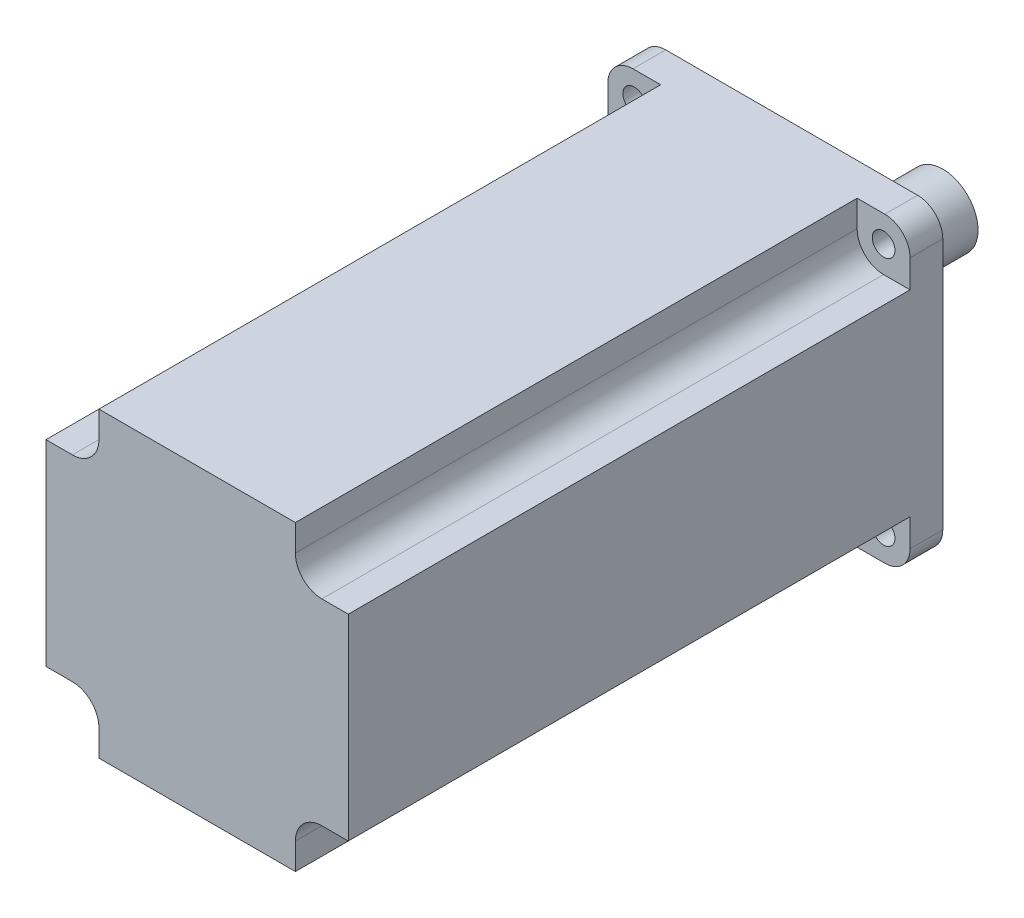
from build123d import *

# Parameters (mm, degrees)
SKETCH1_R      = 2.25
EXTRUDE1_DEPTH = 6.5
EXTRUDE2_DEPTH = 111.5
SKETCH3_R      = 25
EXTRUDE3_DEPTH = 3
SKETCH4_R      = 7
EXTRUDE4_DEPTH = 27


with BuildPart() as part:
    # Sketch1 → Extrude1 (new body)
    with BuildSketch(Plane.XY):
        with BuildLine():
            Line((-25, -30), (25, -30))
            ThreePointArc((25, -30), (28.535533906, -28.535533906), (30, -25))
            Line((30, -25), (30, 25))
            ThreePointArc((30, 25), (28.535533906, 28.535533906), (25, 30))
            Line((25, 30), (-25, 30))
            ThreePointArc((-25, 30), (-28.535533906, 28.535533906), (-30, 25))
            Line((-30, 25), (-30, -25))
            ThreePointArc((-30, -25), (-28.535533906, -28.535533906), (-25, -30))
        make_face()
        with Locations(Location((-24.748737342, 24.748737342, 0), (0, 0, 180))):
            Circle(SKETCH1_R, mode=Mode.SUBTRACT)
        with Locations(Location((-24.748737342, -24.748737342, 0), (0, 0, 180))):
            Circle(SKETCH1_R, mode=Mode.SUBTRACT)
        with Locations(Location((24.748737342, -24.748737342, 0), (0, 0, 180))):
            Circle(SKETCH1_R, mode=Mode.SUBTRACT)
        with Locations(Location((24.748737342, 24.748737342, 0), (0, 0, 180))):
            Circle(SKETCH1_R, mode=Mode.SUBTRACT)
    extrude(amount=EXTRUDE1_DEPTH)

    # Sketch2 → Extrude2 (add)
    with BuildSketch(Plane.XY.offset(6.5)):
        with BuildLine():
            Line((-19.497474683, -30), (19.497474683, -30))
            Line((19.497474683, -30), (19.497474683, -24.748737342))
            ThreePointArc((19.497474683, -24.748737342), (21.035533906, -21.035533906), (24.748737342, -19.497474683))
            Line((24.748737342, -19.497474683), (30, -19.497474683))
            Line((30, -19.497474683), (30, 19.497474683))
            Line((30, 19.497474683), (24.748737342, 19.497474683))
            ThreePointArc((24.748737342, 19.497474683), (21.035533906, 21.035533906), (19.497474683, 24.748737342))
            Line((19.497474683, 24.748737342), (19.497474683, 30))
            Line((19.497474683, 30), (-19.497474683, 30))
            Line((-19.497474683, 30), (-19.497474683, 24.748737342))
            ThreePointArc((-19.497474683, 24.748737342), (-21.035533906, 21.035533906), (-24.748737342, 19.497474683))
            Line((-24.748737342, 19.497474683), (-30, 19.497474683))
            Line((-30, 19.497474683), (-30, -19.497474683))
            Line((-30, -19.497474683), (-24.748737342, -19.497474683))
            ThreePointArc((-24.748737342, -19.497474683), (-21.035533906, -21.035533906), (-19.497474683, -24.748737342))
            Line((-19.497474683, -24.748737342), (-19.497474683, -30))
        make_face()
    extrude(amount=EXTRUDE2_DEPTH)

    # Sketch3 → Extrude3 (add)
    with BuildSketch(Plane(origin=(0, 0, 0), x_dir=(-1, 0, 0), z_dir=(0, 0, -1))):
        Circle(SKETCH3_R)
    extrude(amount=EXTRUDE3_DEPTH)

    # Sketch4 → Extrude4 (add)
    with BuildSketch(Plane(origin=(0, 0, -3), x_dir=(-1, 0, 0), z_dir=(0, 0, -1))):
        Circle(SKETCH4_R)
    extrude(amount=EXTRUDE4_DEPTH)


solid = part.part
